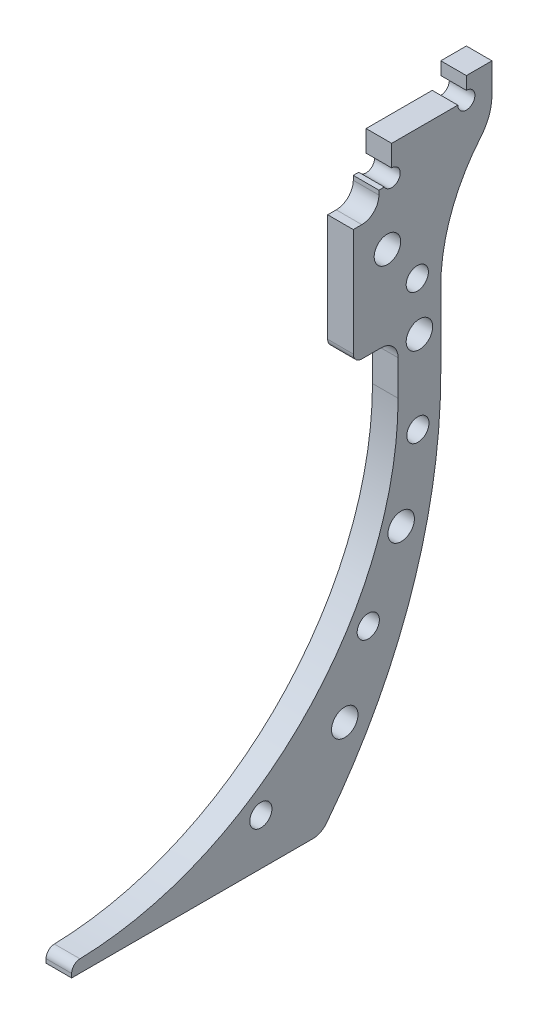
SolidWorks part; units mm, degrees
material "Thornel Mat VMA"
ref_plane "前视基准面" through (0, 0, 0) normal (0, 0, 1) x (1, 0, 0)
ref_plane "上视基准面" through (0, 0, 0) normal (0, 1, 0) x (1, 0, 0)
ref_plane "右视基准面" through (0, 0, 0) normal (1, 0, 0) x (0, 0, -1)
sketch "草图1" plane through (0, 0, 0) normal (1, 0, 0) x (0, 0, -1)
  line L0 (0, 0) -> (0, 48.25) construction
  line L1 (-9.25, 0) -> (-9.25, 19.75)
  line L2 (9.25, 0) -> (9.25, 19.75)
  line L3 (-24, -33.25) -> (-24, -37.75)
  line L4 (9.25, 19.75) -> (19.25, 19.75)
  line L5 (19.25, 19.75) -> (19.25, 0)
  line L6 (-24, -37.75) -> (6.7494, -37.75)
  line L7 (-24, -4.75) -> (-25.4, -4.75)
  line L8 (-25.4, -4.75) -> (-25.4, -14.75)
  line L9 (-25.4, -14.75) -> (-24, -14.75)
  line L10 (-19.25, 0) -> (-19.25, 19.75)
  line L11 (-19.25, 19.75) -> (-9.25, 19.75)
  line L12 (-24, 0) -> (11.1869, -2.1081) construction
  line L13 (-24, 0) -> (10.4888, -7.2859) construction
  line L14 (11.25, 3.1162) -> (11.25, 0) construction
  line L15 (-11.25, 0) -> (-11.25, 3.1162) construction
  line L16 (-24, 0) -> (-11.4381, -2.1822) construction
  line L17 (-24, 0) -> (-13.4117, -7.1029) construction
  line L18 (-24, -33.25) -> (-24, -14.75) construction
  line L19 (14, -37.75) -> (14, -27.25) construction
  line L20 (14, -27.25) -> (19.25, -27.25) construction
  line L21 (-24, 0) -> (-44, 0) construction
  line L22 (11.25, 3.1162) -> (11.1869, -2.1081) construction
  line L23 (10.4888, -7.2859) -> (11.1869, -2.1081) construction
  line L24 (-11.25, 3.1162) -> (-11.4381, -2.1822) construction
  line L25 (-11.4381, -2.1822) -> (-13.4117, -7.1029) construction
  line L26 (-25.4, -9.75) -> (-24, -9.75)
  line L27 (-14.25, 0) -> (-14.25, 19.75)
  line L28 (14.25, 0) -> (14.25, 19.75)
  line L29 (-17.8356, -34.7068) -> (-17.8356, -37.75) construction
  line L30 (-19.25, 19.75) -> (-19.25, 48.25)
  line L31 (-19.25, 48.25) -> (-9.25, 48.25)
  line L32 (19.25, 48.25) -> (19.25, 19.75)
  line L33 (9.25, 19.75) -> (9.25, 48.25)
  line L34 (-9.25, 19.75) -> (-9.25, 48.25)
  line L35 (9.25, 48.25) -> (19.25, 48.25)
  line L36 (-24, 0) -> (-1.8285, -34.25) construction
  line L37 (-24, 0) -> (16.5703, -4.3237) construction
  line L38 (-24, 0) -> (10.7567, -21.3684) construction
  line L39 (16.5703, -4.3237) -> (14.6157, -13.1708) construction
  line L40 (14.6157, -13.1708) -> (10.7567, -21.3684) construction
  line L41 (-14.25, 6.1162) -> (14.25, 6.1162)
  line L42 (5.2389, -39.7) -> (-24, -39.7)
  line L43 (-24, -39.7) -> (-24, -37.75)
  arc A0 (-24, -24) -> (0, 0) centre (-24, 0) ccw construction
  arc A1 (-24, -33.25) -> (9.25, 0) centre (-24, 0) ccw
  arc A2 (-24, -14.75) -> (-9.25, 0) centre (-24, 0) ccw
  arc A3 (5.2389, -39.7) -> (19.25, 0) centre (-44, 0) ccw
  arc A4 (-24, -4.75) -> (-19.25, 0) centre (-24, 0) ccw
  circle A5 centre (11.1869, -2.1081) radius 1.025
  circle A6 centre (10.4888, -7.2859) radius 1.025
  circle A7 centre (9.0331, -12.3036) radius 1.025
  circle A8 centre (6.8516, -17.0511) radius 1.025
  circle A9 centre (3.9925, -21.4239) radius 1.025
  circle A10 centre (0.5183, -25.3262) radius 1.025
  circle A11 centre (-3.4944, -28.672) radius 1.025
  circle A12 centre (-7.9577, -31.388) radius 1.025
  circle A13 centre (11.1869, -2.1081) radius 2.5 construction
  circle A14 centre (10.4888, -7.2859) radius 2.5 construction
  circle A15 centre (11.25, 3.1162) radius 1.025
  circle A16 centre (11.25, 3.1162) radius 2.5 construction
  arc A17 (11.25, 0) -> (-7.9577, -31.388) centre (-24, 0) cw construction
  arc A18 (-11.25, 0) -> (-22.1936, -12.6214) centre (-24, 0) cw construction
  circle A19 centre (-11.4381, -2.1822) radius 1.025
  circle A20 centre (-11.4381, -2.1822) radius 2.5 construction
  circle A21 centre (-13.4117, -7.1029) radius 1.025
  circle A22 centre (-17.2162, -10.7955) radius 1.025
  circle A23 centre (-22.1936, -12.6214) radius 1.025
  circle A25 centre (-11.25, 3.1162) radius 1.025
  circle A26 centre (-11.25, 3.1162) radius 2.5 construction
  circle A27 centre (-13.4117, -7.1029) radius 2.5 construction
  circle A28 centre (8, -29.75) radius 1.55
  circle A29 centre (9.0331, -12.3036) radius 2.5 construction
  circle A30 centre (6.8516, -17.0511) radius 2.5 construction
  circle A31 centre (3.9925, -21.4239) radius 2.5 construction
  circle A32 centre (0.5183, -25.3262) radius 2.5 construction
  circle A33 centre (-3.4944, -28.672) radius 2.5 construction
  circle A34 centre (-7.9577, -31.388) radius 2.5 construction
  circle A35 centre (-17.2162, -10.7955) radius 2.5 construction
  circle A36 centre (-22.1936, -12.6214) radius 2.5 construction
  arc A37 (-24, -9.75) -> (-14.25, 0) centre (-24, 0) ccw
  arc A38 (-24, -38.25) -> (14.25, 0) centre (-24, 0) ccw
  arc A39 (-24, -38.25) -> (14.25, 0) centre (-24, 0) ccw construction
  circle A40 centre (-12.7733, -33.4144) radius 1.025
  circle A41 centre (-17.8356, -34.7068) radius 1.025
  circle A42 centre (-12.7733, -33.4144) radius 2.5 construction
  circle A43 centre (-17.8356, -34.7068) radius 2.5 construction
  circle A44 centre (-21.4, -7.0349) radius 1.3
  circle A45 centre (-16.9174, -2.467) radius 1.55
  arc A48 (-16.9174, -2.467) -> (-21.4, -7.0349) centre (-24, 0) cw construction
  arc A49 (16.5703, -4.3237) -> (-1.8285, -34.25) centre (-24, 0) cw construction
  circle A50 centre (16.5703, -4.3237) radius 1.3
  circle A51 centre (14.6157, -13.1708) radius 1.55
  circle A52 centre (10.7567, -21.3684) radius 1.3
  circle A53 centre (-1.8285, -34.25) radius 1.3
  circle A55 centre (16.75, 5.25) radius 1.55
  circle A56 centre (-16.75, 5.25) radius 1.55
  circle A57 centre (-13, 15.75) radius 1.55
  circle A58 centre (-16.5, 11.05) radius 1.3
  circle A59 centre (16.5, 11.05) radius 1.3
  circle A60 centre (13, 15.75) radius 1.55
  dimension "D1" = 24
  dimension "D2" = 18.5
  dimension "D4" = 10
  dimension "D5" = 1.4
  dimension "D6" = 10
  dimension "D8" = 2.05
  dimension "D10" = 5
  dimension "D11" = 4
  dimension "D13" = 12.75
  dimension "D15" = 3.5
  dimension "D16" = 3.1
  dimension "D18" = 6
  dimension "D23" = 53
  dimension "D24" = 2.6
  dimension "D25" = 3.1
  dimension "D26" = 7.5
  dimension "D33" = 40.8
  dimension "D28" = 6.4
  dimension "D34" = 26
  dimension "D3" = 4.5
  dimension "D7" = 8.5
  dimension "D9" = 35.25
  dimension "D12" = 24
  dimension "D14" = 24.5
  dimension "D17" = 8
  dimension "D19" = 2.5
  dimension "D20" = 20
  dimension "D21" = 5
  dimension "D27" = 4
  dimension "D29" = 2.5
  dimension "D30" = 14.5
  dimension "D31" = 32
  dimension "D32" = 1.95
  dimension "D35" = 51
  dimension "D36" = 3
  dimension "D37" = 33
  dimension "D38" = 5.8
  dimension "D39" = 4
  dimension "D22" = 5
extrude "凸台-拉伸1" add sketch "草图1" along normal blind 3 contours A38 L6 A3 L5 L4 L28 A55 A53 A52 A51 A50 A28 | L2 L41 L28 L4 | L42 A3 L6 L43
sketch "草图2" plane through (3, 0, 0) normal (1, 0, 0) x (0, 0, -1)
  line L0 (9.25, 6.1162) -> (9.25, 19.75) construction
  line L1 (9.25, 19.75) -> (19.25, 19.75) construction
  line L2 (9.25, 6.1162) -> (9.25, 19.75)
  line L3 (12, 19.75) -> (19.25, 19.75)
  line L4 (9.25, 6.1162) -> (9, 6.1162)
  line L5 (9, 6.1162) -> (9, 19.75)
  line L6 (22.25, 28.75) -> (25.25, 28.75)
  line L8 (22.25, 28.75) -> (22.25, 27.25)
  line L9 (21.25, 26.25) -> (13.5, 26.25)
  line L10 (13.5, 26.25) -> (13.5, 23.75)
  line L11 (12.634, 22.25) -> (12, 22.25)
  line L12 (12, 22.25) -> (12, 19.75)
  line L13 (9.25, 19.75) -> (9, 19.75)
  line L14 (19.25, 19.75) -> (19.25, 0) construction
  line L15 (19.25, 19.75) -> (19.25, 8.8001)
  line L16 (25.25, 28.75) -> (25.25, 25.25)
  arc A0 (23.9467, 21.6767) -> (19.25, 8.8001) centre (39.25, 8.8001) ccw
  arc A1 (12.634, 22.25) -> (13.5, 23.75) centre (13.5, 22.75) ccw
  arc A2 (21.25, 26.25) -> (22.25, 27.25) centre (22.25, 26.25) ccw
  arc A3 (25.25, 25.25) -> (23.9467, 21.6767) centre (19.7, 25.25) cw
  dimension "D2" = 20
  dimension "D3" = 1
  dimension "D11" = 5.55
  dimension "D1" = 0.25
  dimension "D4" = 6
  dimension "D5" = 2.5
  dimension "D6" = 13.5
  dimension "D7" = 1.5
  dimension "D8" = 6.5
  dimension "D9" = 3
  dimension "D10" = 2.5
  dimension "D12" = 3.5
  dimension "D13" = 0.5
extrude "凸台-拉伸2" add sketch "草图2" against normal through all
fillet "R2 圆角1" radius 2 3 edges at (1.5, 6.1162, -14.25) (1.5, 19.75, -12) (1.5, -39.7, -5.2389)
fillet "R1 圆角2" radius 1 2 edges at (1.5, -38.25, 24) (1.5, 6.1162, -9)
